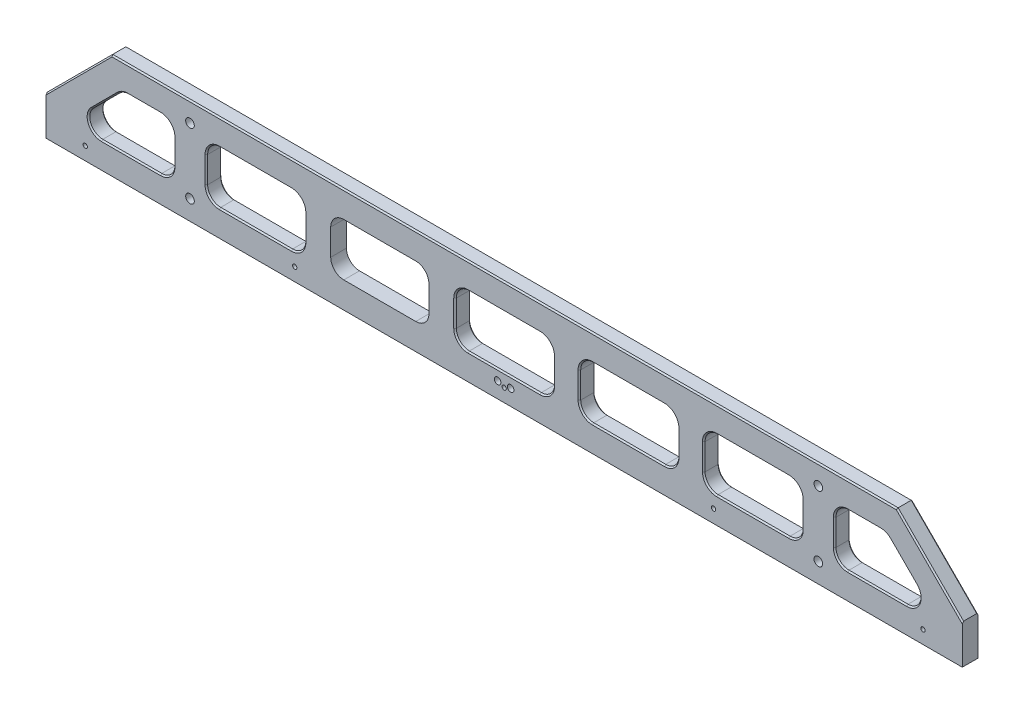
SolidWorks part; units mm, degrees
ref_plane "前视基准面" through (0, 0, 0) normal (0, 0, 1) x (1, 0, 0)
ref_plane "上视基准面" through (0, 0, 0) normal (0, 1, 0) x (1, 0, 0)
ref_plane "右视基准面" through (0, 0, 0) normal (1, 0, 0) x (0, 0, -1)
ref_plane "基准面4" through (0, 0, 0) normal (0, 0, -1) x (-1, 0, 0)
sketch "草图1" plane through (0, 0, 0) normal (0, 0, -1) x (-1, 0, 0)
  line L0 (-300, 32.6421) -> (-350, -17.3579)
  line L1 (-350, -17.3579) -> (-350, -47.3579)
  line L2 (-350, -47.3579) -> (350, -47.3579)
  line L3 (350, -47.3579) -> (350, -17.3579)
  line L4 (350, -17.3579) -> (300, 32.6421)
  line L5 (300, 32.6421) -> (-300, 32.6421)
extrude "凸台-拉伸1" add sketch "草图1" against normal blind 12
sketch "草图2" plane through (0, 0, 0) normal (0, 0, -1) x (-1, 0, 0)
  line L0 (132.5, -27.3579) -> (132.5, 12.6421)
  line L1 (132.5, 12.6421) -> (57.5, 12.6421)
  line L2 (57.5, 12.6421) -> (57.5, -27.3579)
  line L3 (57.5, -27.3579) -> (132.5, -27.3579)
extrude "切除-拉伸1" cut sketch "草图2" against normal through all
sketch "草图3" plane through (0, 0, 0) normal (0, 0, -1) x (-1, 0, 0)
  line L0 (-291.7157, 12.6421) -> (-314.6447, -10.2868)
  line L1 (-307.5736, -27.3579) -> (-252.5, -27.3579)
  line L2 (-252.5, -27.3579) -> (-252.5, 12.6421)
  line L3 (-252.5, 12.6421) -> (-291.7157, 12.6421)
  arc A0 (-314.6447, -10.2868) -> (-307.5736, -27.3579) centre (-307.5736, -17.3579) ccw
extrude "切除-拉伸2" cut sketch "草图3" against normal through all
sketch "草图4" plane through (0, 0, 0) normal (0, 0, -1) x (-1, 0, 0)
  line L0 (37.5, 12.6421) -> (-37.5, 12.6421)
  line L1 (-37.5, 12.6421) -> (-37.5, -27.3579)
  line L2 (-37.5, -27.3579) -> (37.5, -27.3579)
  line L3 (37.5, -27.3579) -> (37.5, 12.6421)
extrude "切除-拉伸3" cut sketch "草图4" against normal through all
sketch "草图5" plane through (0, 0, 0) normal (0, 0, -1) x (-1, 0, 0)
  line L0 (-227.5, 12.6421) -> (-227.5, -27.3579)
  line L1 (-227.5, -27.3579) -> (-152.5, -27.3579)
  line L2 (-152.5, -27.3579) -> (-152.5, 12.6421)
  line L3 (-152.5, 12.6421) -> (-227.5, 12.6421)
extrude "切除-拉伸4" cut sketch "草图5" against normal through all
sketch "草图6" plane through (0, 0, 0) normal (0, 0, -1) x (-1, 0, 0)
  line L0 (227.5, -27.3579) -> (227.5, 12.6421)
  line L1 (227.5, 12.6421) -> (152.5, 12.6421)
  line L2 (152.5, 12.6421) -> (152.5, -27.3579)
  line L3 (152.5, -27.3579) -> (227.5, -27.3579)
extrude "切除-拉伸5" cut sketch "草图6" against normal through all
sketch "草图7" plane through (0, 0, 0) normal (0, 0, -1) x (-1, 0, 0)
  line L0 (291.7157, 12.6421) -> (252.5, 12.6421)
  line L1 (252.5, 12.6421) -> (252.5, -27.3579)
  line L2 (252.5, -27.3579) -> (307.5736, -27.3579)
  line L3 (314.6447, -10.2868) -> (291.7157, 12.6421)
  arc A0 (307.5736, -27.3579) -> (314.6447, -10.2868) centre (307.5736, -17.3579) ccw
extrude "切除-拉伸6" cut sketch "草图7" against normal through all
sketch "草图8" plane through (0, 0, 12) normal (0, 0, 1) x (1, 0, 0)
  line L0 (132.5, -27.3579) -> (132.5, 12.6421)
  line L1 (132.5, 12.6421) -> (57.5, 12.6421)
  line L2 (57.5, 12.6421) -> (57.5, -27.3579)
  line L3 (57.5, -27.3579) -> (132.5, -27.3579)
extrude "切除-拉伸7" cut sketch "草图8" against normal through all
hole_wizard "Ø3.3 (3.3) 直径孔1" positions "草图10" profile "草图9" hole size "Ø3.3" standard "ANSI Metric"
sketch "草图10" plane through (0, 0, 0) normal (0, 0, -1) x (-1, 0, 0)
  point P0 (-320, -37.3579)
  point P1 (-160, -37.3579)
  point P2 (0, -37.3579)
  point P3 (160, -37.3579)
  point P4 (320, -37.3579)
sketch "草图9" plane through (320, -37.3579, 0) normal (1, 0, 0) x (0, 1, 0)
  line L0 (0, 0) -> (0, 12)
  line L1 (0, 12) -> (1.65, 12)
  line L2 (1.65, 12) -> (1.65, 0)
  line L5 (1.65, 0) -> (0, 0)
  line L11 (0, -6.35) -> (0, 107.95) construction
  dimension "通孔孔直径" = 3.3
  dimension "通孔孔深度" = 12
hole_wizard "Ø5.0 (5) 直径孔1" positions "草图12" profile "草图11" hole size "Ø5.0" standard "ANSI Metric"
sketch "草图12" plane through (0, 0, 12) normal (0, 0, 1) x (1, 0, 0)
  point P0 (5, -35.3579)
  point P1 (-5, -35.3579)
sketch "草图11" plane through (5, -35.3579, 12) normal (1, 0, 0) x (0, -1, 0)
  line L0 (0, 0) -> (0, 12)
  line L1 (0, 12) -> (2.5, 12)
  line L2 (2.5, 12) -> (2.5, 0)
  line L5 (2.5, 0) -> (0, 0)
  line L11 (0, -6.35) -> (0, 107.95) construction
  dimension "通孔孔直径" = 5
  dimension "通孔孔深度" = 12
hole_wizard "M6 六角头螺栓的柱形沉头孔1" positions "草图14" profile "草图13" counterbore size "M6" standard "ANSI Metric"
sketch "草图14" plane through (0, 0, 0) normal (0, 0, -1) x (-1, 0, 0)
  point P0 (-240, 17.6421)
  point P1 (-240, -32.3579)
  point P2 (240, -32.3579)
  point P3 (240, 17.6421)
sketch "草图13" plane through (240, 17.6421, 0) normal (1, 0, 0) x (0, 1, 0)
  line L0 (0, 0) -> (0, 12)
  line L1 (0, 12) -> (3.3, 12)
  line L3 (3.3, 12) -> (3.3, 6.4)
  line L4 (3.3, 6.4) -> (5.5, 6.4)
  line L5 (5.5, 6.4) -> (5.5, 0)
  line L7 (5.5, 0) -> (0, 0)
  line L11 (0, -6.35) -> (0, 107.95) construction
  dimension "通孔孔直径" = 6.6
  dimension "通孔孔深度" = 12
  dimension "柱形沉头孔直径" = 11
  dimension "柱形沉头孔深度" = 6.4
hole_wizard "Ø5.0 (5) 直径孔2" positions "草图16" profile "草图15" hole size "Ø5.0" standard "ANSI Metric"
sketch "草图16" plane through (0, -47.3579, 0) normal (0, -1, 0) x (-1, 0, 0)
  point P0 (290, -6)
  point P1 (174, -6)
  point P2 (58, -6)
  point P3 (-58, -6)
  point P4 (-290, -6)
  point P5 (-174, -6)
sketch "草图15" plane through (-290, -47.3579, 6) normal (1, 0, 0) x (0, 0, -1)
  line L0 (0, 0) -> (0, 16.5022)
  line L1 (0, 16.5022) -> (2.5, 15)
  line L2 (2.5, 15) -> (2.5, 0)
  line L5 (2.5, 0) -> (0, 0)
  line L10 (0, 16.5022) -> (-2.5, 15) construction
  line L11 (0, -6.35) -> (0, 107.95) construction
  dimension "孔直径" = 5
  dimension "孔深度" = 15
  dimension "导头角度" = 118
fillet "圆角1" radius 10 26 edges at (-132.5, -27.3579, 6) (-57.5, 12.6421, 6) (-57.5, -27.3579, 6) (-132.5, 12.6421, 6) (37.5, 12.6421, 6) (-291.7157, 12.6421, 6) (-152.5, -27.3579, 6) (132.5, -27.3579, 6) (-37.5, -27.3579, 6) (252.5, -27.3579, 6) (-227.5, 12.6421, 6) (252.5, 12.6421, 6) (291.7157, 12.6421, 6) (-37.5, 12.6421, 6) (152.5, -27.3579, 6) (37.5, -27.3579, 6) (152.5, 12.6421, 6) (-152.5, 12.6421, 6) (227.5, 12.6421, 6) (-227.5, -27.3579, 6) (227.5, -27.3579, 6) (-252.5, -27.3579, 6) (57.5, -27.3579, 6) (-252.5, 12.6421, 6) (57.5, 12.6421, 6) (132.5, 12.6421, 6)
chamfer "倒角1" distance 1 angle 45 102 edges at (-190, -27.3579, 12) (-224.5711, -24.4289, 12) (-155.4289, -24.4289, 12) (-227.5, -7.3579, 12) (-152.5, -7.3579, 12) (-224.5711, 9.7132, 12) (-155.4289, 9.7132, 12) (-190, 12.6421, 12) (95, 12.6421, 0) (60.4289, 9.7132, 0) (129.5711, 9.7132, 0) (57.5, -7.3579, 0) (132.5, -7.3579, 0) (60.4289, -24.4289, 0) (129.5711, -24.4289, 0) (95, -27.3579, 0) (316.8124, -21.1847, 0) (304.6447, -0.2868, 0) (285.0368, -27.3579, 0) (291.4004, 11.8809, 0) (255.4289, -24.4289, 0) (275.0368, 12.6421, 0) (252.5, -7.3579, 0) (255.4289, 9.7132, 0) (37.5, -7.3579, 0) (34.5711, -24.4289, 0) (34.5711, 9.7132, 0) (0, -27.3579, 0) (0, 12.6421, 0) (-34.5711, -24.4289, 0) (-34.5711, 9.7132, 0) (-37.5, -7.3579, 0) (37.5, -7.3579, 12) (34.5711, -24.4289, 12) (34.5711, 9.7132, 12) (0, -27.3579, 12) (0, 12.6421, 12) (-34.5711, -24.4289, 12) (-34.5711, 9.7132, 12) (-37.5, -7.3579, 12) (-316.8124, -21.1847, 12) (-304.6447, -0.2868, 12) (-285.0368, -27.3579, 12) (-291.4004, 11.8809, 12) (-255.4289, -24.4289, 12) (-275.0368, 12.6421, 12) (-252.5, -7.3579, 12) (-255.4289, 9.7132, 12) (224.5711, -24.4289, 0) (227.5, -7.3579, 0) (190, -27.3579, 0) (224.5711, 9.7132, 0) (155.4289, -24.4289, 0) (190, 12.6421, 0) (152.5, -7.3579, 0) (155.4289, 9.7132, 0) (-224.5711, 9.7132, 0) (-227.5, -7.3579, 0) (-190, 12.6421, 0) (-224.5711, -24.4289, 0) (-155.4289, 9.7132, 0) (-190, -27.3579, 0) (-152.5, -7.3579, 0) (-155.4289, -24.4289, 0) (255.4289, 9.7132, 12) (275.0368, 12.6421, 12) (252.5, -7.3579, 12) (291.4004, 11.8809, 12) (255.4289, -24.4289, 12) (304.6447, -0.2868, 12) (285.0368, -27.3579, 12) (316.8124, -21.1847, 12) (-252.5, -7.3579, 0) (-255.4289, 9.7132, 0) (-255.4289, -24.4289, 0) (-275.0368, 12.6421, 0) (-285.0368, -27.3579, 0) (-291.4004, 11.8809, 0) (-316.8124, -21.1847, 0) (-304.6447, -0.2868, 0) (-325, 7.6421, 12) (325, 7.6421, 12) (0, 32.6421, 12) (325, 7.6421, 0) (0, 32.6421, 0) (-325, 7.6421, 0) (224.5711, 9.7132, 12) (227.5, -7.3579, 12) (190, 12.6421, 12) (224.5711, -24.4289, 12) (155.4289, 9.7132, 12) (190, -27.3579, 12) (152.5, -7.3579, 12) (155.4289, -24.4289, 12) (95, 12.6421, 12) (129.5711, 9.7132, 12) (60.4289, 9.7132, 12) (132.5, -7.3579, 12) (57.5, -7.3579, 12) (129.5711, -24.4289, 12) (60.4289, -24.4289, 12) (95, -27.3579, 12)
